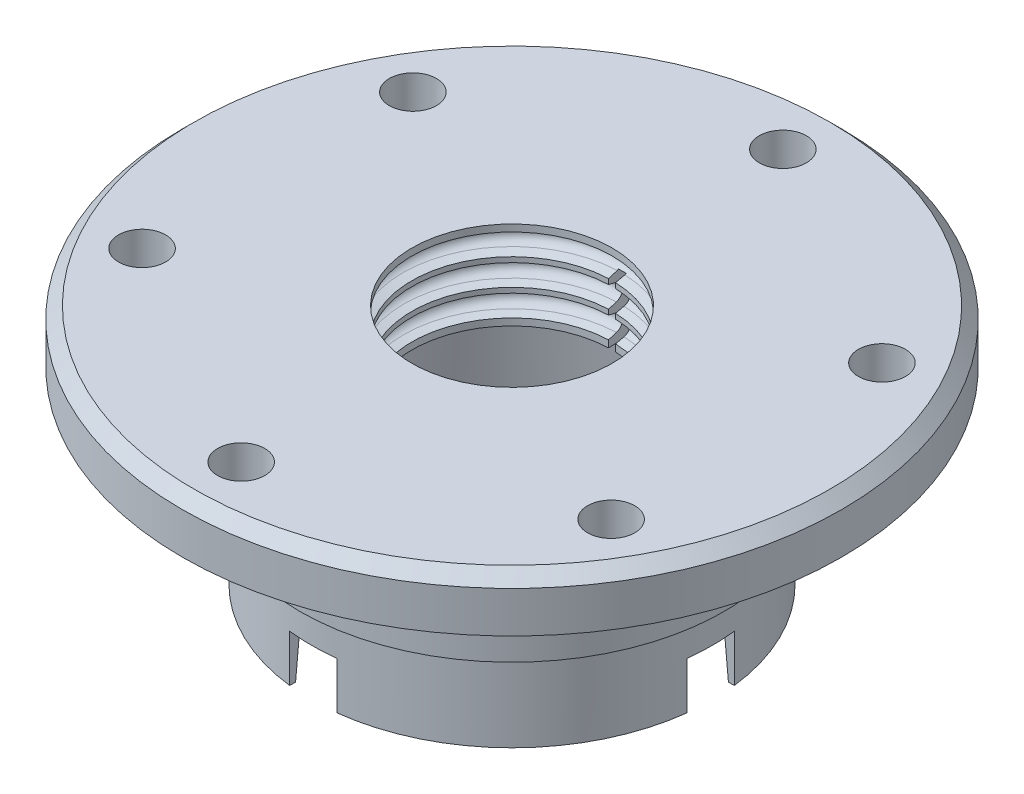
SolidWorks part; units mm, degrees
ref_plane "Front" through (0, 0, 0) normal (0, 0, 1) x (1, 0, 0)
ref_plane "Top" through (0, 0, 0) normal (0, 1, 0) x (1, 0, 0)
ref_plane "Right" through (0, 0, 0) normal (1, 0, 0) x (0, 0, -1)
sketch "Sketch1" plane through (0, 0, 0) normal (0, 0, 1) x (1, 0, 0)
  line L0 (-34, 0) -> (-34, 14)
  line L1 (-34, 14) -> (-36, 14)
  line L2 (-36, 14) -> (-36, 30)
  line L3 (-34, 32) -> (-56, 32)
  line L4 (-56, 32) -> (-56.0098, 32.0175)
  line L5 (-56, 39) -> (-54, 41)
  line L6 (-56, 32) -> (-56, 39)
  line L7 (-54, 41) -> (-17, 41)
  line L8 (-34, 0) -> (-33, 0)
  line L9 (-17, 36.1791) -> (-17, 35.3137) construction
  line L10 (-17, 26) -> (-26.0093, 26)
  line L11 (-30.9875, 21.4667) -> (-33, 0)
  line L12 (-36, 30) -> (-34, 30)
  line L13 (-34, 30) -> (-34, 32)
  line L14 (-6.8412, 38) -> (-2, 38) construction
  line L15 (-6.8412, 33.5) -> (-18, 33.5) construction
  line L16 (-6.8412, 29) -> (-18, 29) construction
  line L17 (-18, 48.7019) -> (-18, 39.5) construction
  line L18 (-17, 36.1863) -> (-17, 36.1791)
  line L19 (-18, 38.2829) -> (-18, 36.5) construction
  line L20 (-18.5251, 34.9051) -> (-17, 35.3137)
  line L21 (-18.3882, 32.0511) -> (-17, 31.6791)
  line L22 (-18.3882, 30.4489) -> (-17, 30.8209)
  line L23 (-18.3882, 27.5511) -> (-17, 27.1791)
  line L24 (-18, 36.5) -> (-18, 16.0195) construction
  line L25 (-17, 43.4667) -> (-17, 39.8209) construction
  line L26 (-17, 41) -> (-17, 39.8209)
  line L27 (-17, 36.1791) -> (-17, 35.3137)
  line L28 (-17, 31.6791) -> (-17, 30.8209) construction
  line L29 (-17, 31.6791) -> (-17, 30.8209)
  line L30 (-17, 27.1791) -> (-17, 26)
  line L31 (-17, 27.1791) -> (-17, 19.5738) construction
  line L32 (0, 0) -> (0, 19.5738) construction
  line L33 (-18.3882, 39.4489) -> (-17, 39.8209)
  line L34 (-18.5251, 36.5949) -> (-17, 36.1863)
  line L35 (-18, 38) -> (-18.5251, 38) construction
  line L36 (-18, 38) -> (-23.8687, 38) construction
  arc A0 (-26.0093, 26) -> (-30.9875, 21.4667) centre (-26.0093, 21) ccw
  arc A1 (-18.3882, 39.4489) -> (-18.5251, 36.5949) centre (-18, 38) ccw
  arc A2 (-18.5251, 34.9051) -> (-18.3882, 32.0511) centre (-18, 33.5) ccw
  arc A3 (-18.3882, 30.4489) -> (-18.3882, 27.5511) centre (-18, 29) ccw
  point P9 (-56, 41)
  dimension "D6" = 5
  dimension "D18" = 37
  dimension "D19" = 3
  dimension "D20" = 3
  dimension "D21" = 15
  dimension "D17" = 30
  dimension "D10" = 3
  dimension "D1" = 14
  dimension "D2" = 2
  dimension "D3" = 34
  dimension "D4" = 2
  dimension "D5" = 22
  dimension "D7" = 3
  dimension "D8" = 9
  dimension "D9" = 1
  dimension "D11" = 4.5
  dimension "D13" = 0
  dimension "D14" = 2
  dimension "D15" = 16
  dimension "D16" = 4.5
  dimension "D22" = 30
  dimension "D23" = 15
  dimension "D24" = 30
  dimension "D25" = 15
  dimension "D26" = 1
revolve "Revolve1" add sketch "Sketch1" angle 360 about L32
sketch "Sketch3" plane through (0, 0, 0) normal (1, 0, 0) x (0, 0, -1)
  line L0 (-17, 32.7164) -> (-17, 26)
  line L1 (-18, 38) -> (-17, 38)
  line L3 (-17, 38) -> (-17, 32.7164)
  line L4 (0, 0) -> (0, 52.8375) construction
  line L5 (18, 38) -> (17, 38)
  line L6 (-21, 38) -> (-24.2154, 26)
  line L7 (-24.2154, 26) -> (-17, 26)
  line L8 (24.2154, 26) -> (17, 26)
  line L9 (17, 32.7164) -> (17, 26)
  line L10 (17, 38) -> (17, 32.7164)
  line L11 (21, 38) -> (24.2154, 26)
  arc A0 (-21, 38) -> (-18, 38) centre (-19.5, 38) ccw
  arc A1 (21, 38) -> (18, 38) centre (19.5, 38) cw
  dimension "D5" = 3
  dimension "D1" = 37
revolve "Cut-Revolve1" cut sketch "Sketch3" angle 4 mid plane about L4
sketch "Sketch4" plane through (0, 0, 0) normal (1, 0, 0) x (0, 0, -1)
  line L0 (-34, 0) -> (34, 0) construction
  line L1 (12.5865, 0) -> (50.3459, 0)
  line L2 (12.5865, 0) -> (12.5865, 8)
  line L3 (12.5865, 8) -> (50.3459, 8)
  line L4 (50.3459, 0) -> (50.3459, 8)
  line L5 (0, 0) -> (0, 50.8648) construction
  line L6 (-12.5865, 0) -> (-12.5865, 8)
  line L7 (-12.5865, 0) -> (-50.3459, 0)
  line L8 (-12.5865, 8) -> (-50.3459, 8)
  line L9 (-50.3459, 0) -> (-50.3459, 8)
  dimension "D1" = 8
extrude "Cut-Extrude1" cut sketch "Sketch4" against normal mid plane 8
sketch "Sketch5" plane through (0, 0, 0) normal (0, 0, 1) x (1, 0, 0)
  line L0 (4, 0) -> (34, 0) construction
  line L1 (10.8558, 0) -> (55.8524, 0)
  line L2 (10.8558, 0) -> (10.8558, 8)
  line L3 (10.8558, 8) -> (55.8524, 8)
  line L4 (55.8524, 0) -> (55.8524, 8)
  line L5 (0, 0) -> (0, 46.7742) construction
  line L6 (-10.8558, 0) -> (-55.8524, 0)
  line L7 (-55.8524, 0) -> (-55.8524, 8)
  line L8 (-10.8558, 8) -> (-55.8524, 8)
  line L9 (-10.8558, 0) -> (-10.8558, 8)
  dimension "D1" = 8
extrude "Cut-Extrude2" cut sketch "Sketch5" against normal mid plane 8
sketch "Sketch6" plane through (0, 0, 0) normal (0, -1, 0) x (1, 0, 0)
  line L0 (0, 0) -> (0, 59.4681) construction
  line L1 (0, 0) -> (66.9707, 38.6656) construction
  line L2 (0, 0) -> (-56.9215, 32.8636) construction
  line L3 (0, 0) -> (78.971, 0) construction
  circle A0 centre (-39.8372, -23) radius 4
  circle A1 centre (0, 46) radius 4
  circle A2 centre (39.8372, 23) radius 4
  circle A3 centre (-39.8372, 23) radius 4
  circle A4 centre (0, -46) radius 4
  circle A5 centre (39.8372, -23) radius 4
  dimension "D4" = 8
  dimension "D5" = 8
  dimension "D1" = 60
  dimension "D2" = 60
extrude "Cut-Extrude3" cut sketch "Sketch6" against normal blind 65
scale "Scale 1" bodies to scale 105 scale about centroid uniform scaling yes scale factor 1.875
